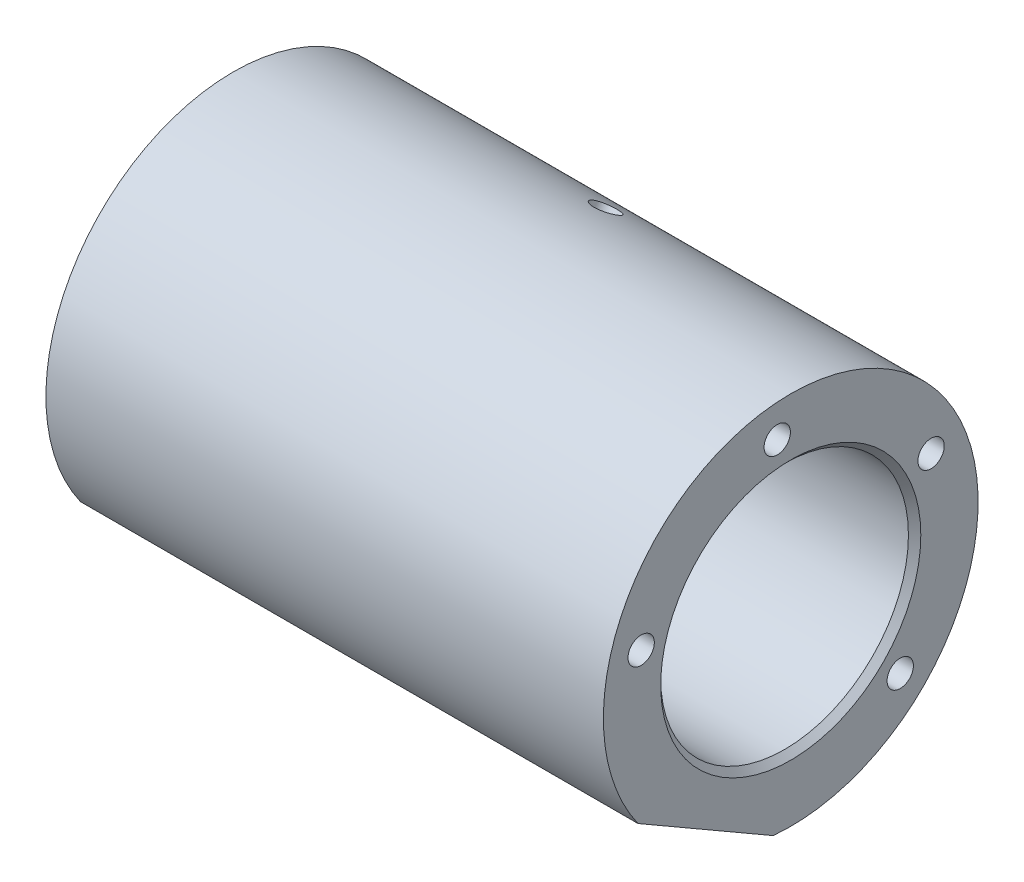
from build123d import *

# Parameters (mm, degrees)
SKETCH1_R               = 60.5
SKETCH1_R_2             = 40
BOSS_EXTRUDE1_DEPTH     = 90
CUT_EXTRUDE1_DEPTH      = 125.179305844
CUT_EXTRUDE1_DEPTH_BACK = 125.179305844
SKETCH6_W               = 4.25
SKETCH6_H               = 82.644536929
M10_TAPPED_HOLE2_D      = 8.5
M10_TAPPED_HOLE2_DEPTH  = 32
M10_TAPPED_HOLE2_TIP    = 2.553657631
CHAMFER1_SIZE           = 2


with BuildPart() as part:
    # Sketch1 → Boss-Extrude1 (new, symmetric)
    with BuildSketch(Plane(origin=(0, 0, 0), x_dir=(0, 0, -1), z_dir=(1, 0, 0))):
        with Locations(Location((0, 0, 0), (0, 0, 180))):
            Circle(SKETCH1_R)
        with Locations(Location((0, 0, 0), (0, 0, 180))):
            Circle(SKETCH1_R_2, mode=Mode.SUBTRACT)
    extrude(amount=BOSS_EXTRUDE1_DEPTH, both=True)

    # Sketch5 → Cut-Extrude1 (cut, two sides: drawn at the far end of the back side and taken through both)
    with BuildSketch(Plane(origin=(0, 0, 0), x_dir=(0, 0, -1), z_dir=(1, 0, 0)).offset(-CUT_EXTRUDE1_DEPTH_BACK)):
        with BuildLine():
            Line((-49.327448316, -35.029314047), (-5.672551684, -60.233480369))
            ThreePointArc((-5.672551684, -60.233480369), (-30.25, -52.394536929), (-49.327448316, -35.029314047))
        make_face()
    extrude(amount=CUT_EXTRUDE1_DEPTH + CUT_EXTRUDE1_DEPTH_BACK, mode=Mode.SUBTRACT)

    # Sketch6 → M10 Tapped Hole1 (revolve, cut)
    with BuildSketch(Plane(origin=(0, 0, 0), x_dir=(0, -0.500000000000001, -0.8660254037844382), z_dir=(1, 0, 0))):
        with Locations((2.125, 41.322268465)):
            Rectangle(SKETCH6_W, SKETCH6_H)
    revolve(axis=Axis((0, -5.499261314, 3.175), (0, 0.866025403784438, -0.500000000000001)), mode=Mode.SUBTRACT)

    # M10 Tapped Hole2
    with Locations(Plane(origin=(90, 0, 0), x_dir=(0, 0, -1), z_dir=(1, 0, 0))):
        with Locations((-4.357787137, 49.809734905), (45.315389352, 21.130913087), (35.355339059, -35.355339059), (-48.296291314, 12.940952255)):
            Hole(M10_TAPPED_HOLE2_D / 2, depth=M10_TAPPED_HOLE2_DEPTH)
            with Locations((0, 0, -(M10_TAPPED_HOLE2_DEPTH + M10_TAPPED_HOLE2_TIP / 2))):  # 118° drill point
                Cone(0, M10_TAPPED_HOLE2_D / 2, M10_TAPPED_HOLE2_TIP, mode=Mode.SUBTRACT)

    # Chamfer1
    chamfer1_edges = [part.edges().sort_by_distance(p)[0] for p in [
        (-90, 0, -40),
        (90, 0, -40),
    ]]
    chamfer(chamfer1_edges, length=CHAMFER1_SIZE)


solid = part.part
